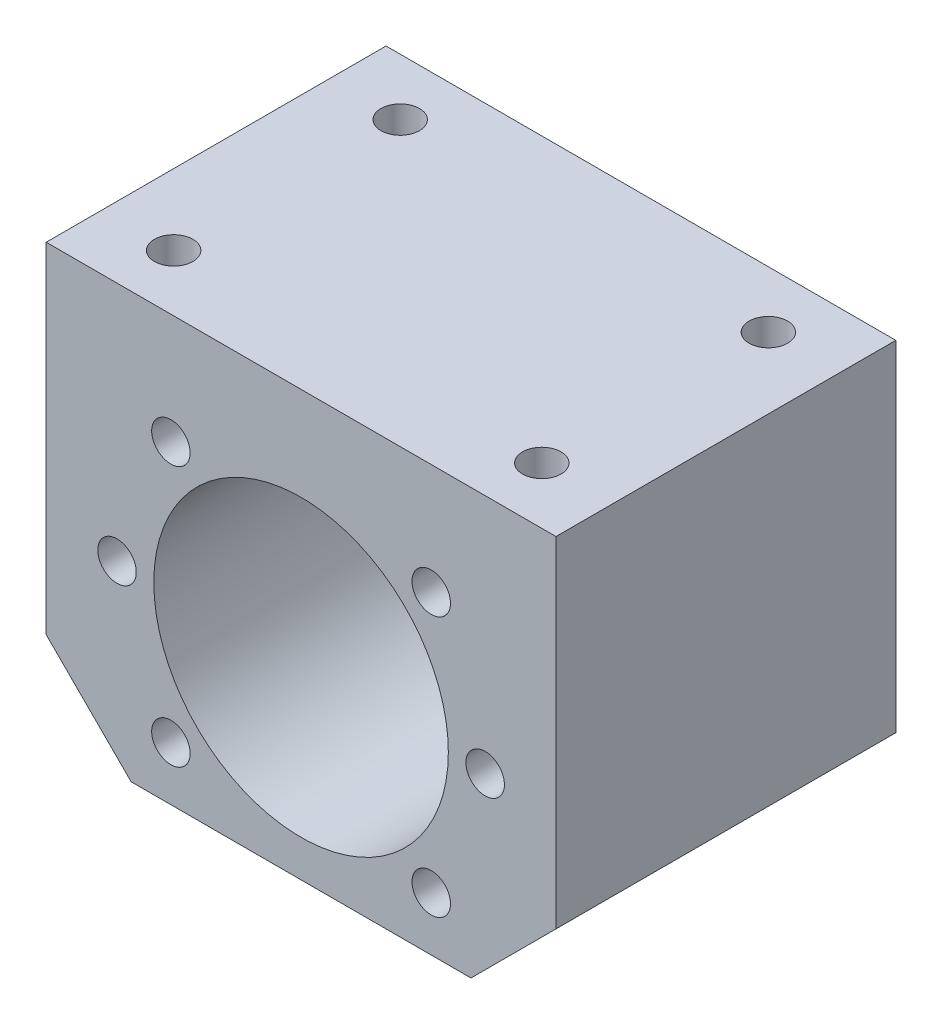
SolidWorks part; units mm, degrees
material "6061 合金"
ref_plane "前视基准面" through (0, 0, 0) normal (0, 0, 1) x (1, 0, 0)
ref_plane "上视基准面" through (0, 0, 0) normal (0, 1, 0) x (1, 0, 0)
ref_plane "右视基准面" through (0, 0, 0) normal (1, 0, 0) x (0, 0, -1)
sketch "草图1" plane through (0, 0, 0) normal (0, 0, 1) x (1, 0, 0)
  line L1 (45, -32.5) -> (-45, -32.5)
  line L2 (45, -32.5) -> (45, 42.5)
  line L3 (45, 42.5) -> (-45, 42.5)
  line L4 (-45, -32.5) -> (-45, 42.5)
  line L5 (45, -32.5) -> (-45, 42.5) construction
  line L6 (45, 42.5) -> (-45, -32.5) construction
  circle A1 centre (0, 0) radius 26
  point P1 (0, 5)
  dimension "D1" = 52
  dimension "D2" = 90
  dimension "D3" = 5
  dimension "D4" = 75
extrude "凸台-拉伸1" add sketch "草图1" along normal mid plane 60
sketch "草图2" plane through (0, 0, 30) normal (0, 0, 1) x (1, 0, 0)
  circle A0 centre (0, 0) radius 32.5
  point P3 (-32.5, 0)
  point P7 (-22.981, 22.981)
  point P8 (0, 32.5)
  point P9 (22.981, 22.981)
  point P10 (32.5, 0)
  point P11 (22.981, -22.981)
  point P12 (0, -32.5)
  point P13 (-22.981, -22.981)
  point P14 (0, 0)
  dimension "D1" = 65
  dimension "D2" = 8
hole_wizard "M8 螺纹孔1" positions "3D草图1" profile "草图3" tap size "M8" standard "GB"
sketch3d "3D草图1"
  point P0 (-32.5, 0, 30)
  point P3 (-22.981, 22.981, 30)
  point P6 (-22.981, -22.981, 30)
  point P9 (22.981, -22.981, 30)
  point P12 (32.5, 0, 30)
  point P15 (22.981, 22.981, 30)
sketch "草图3" plane through (-32.5, 0, 30) normal (1, 0, 0) x (0, -1, 0)
  line L0 (0, 0) -> (0, 21.7929)
  line L1 (0, 21.7929) -> (3.4, 19.75)
  line L2 (3.4, 19.75) -> (3.4, 0)
  line L5 (3.4, 0) -> (0, 0)
  line L10 (0, 21.7929) -> (-3.4, 19.75) construction
  line L11 (0, -6.35) -> (0, 107.95) construction
  dimension "螺纹孔钻头直径" = 6.8
  dimension "螺纹孔钻头深度" = 19.75
  dimension "导头角度" = 118
cosmetic thread "孔螺蚊线1" parameters "D1"=16, "D2"=8
cosmetic thread "孔螺蚊线2" parameters "D1"=16, "D2"=8
cosmetic thread "孔螺蚊线3" parameters "D1"=16, "D2"=8
cosmetic thread "孔螺蚊线4" parameters "D1"=16, "D2"=8
cosmetic thread "孔螺蚊线5" parameters "D1"=16, "D2"=8
cosmetic thread "孔螺蚊线6" parameters "D1"=16, "D2"=8
chamfer "倒角1" distance 15 angle 45 2 edges at (45, -32.5, 0) (-45, -32.5, 0)
sketch "草图4" plane through (0, 42.5, 0) normal (0, 1, 0) x (1, 0, 0)
  line L1 (32.5, -20) -> (-32.5, -20)
  line L2 (32.5, -20) -> (32.5, 20)
  line L3 (32.5, 20) -> (-32.5, 20)
  line L4 (-32.5, -20) -> (-32.5, 20)
  line L5 (32.5, -20) -> (-32.5, 20) construction
  line L6 (32.5, 20) -> (-32.5, -20) construction
  point P0 (0, 0)
  dimension "D1" = 65
  dimension "D2" = 40
hole_wizard "M8 螺纹孔2" positions "3D草图2" profile "草图5" tap size "M8" standard "GB"
sketch3d "3D草图2"
  point P2 (32.5, 42.5, -20)
  point P5 (32.5, 42.5, 20)
  point P8 (-32.5, 42.5, 20)
  point P11 (-32.5, 42.5, -20)
sketch "草图5" plane through (32.5, 42.5, -20) normal (1, 0, 0) x (0, 0, 1)
  line L0 (0, 0) -> (0, 21.7929)
  line L1 (0, 21.7929) -> (3.4, 19.75)
  line L2 (3.4, 19.75) -> (3.4, 0)
  line L5 (3.4, 0) -> (0, 0)
  line L10 (0, 21.7929) -> (-3.4, 19.75) construction
  line L11 (0, -6.35) -> (0, 107.95) construction
  dimension "螺纹孔钻头直径" = 6.8
  dimension "螺纹孔钻头深度" = 19.75
  dimension "导头角度" = 118
cosmetic thread "孔螺蚊线7" parameters "D1"=16, "D2"=8
cosmetic thread "孔螺蚊线8" parameters "D1"=16, "D2"=8
cosmetic thread "孔螺蚊线9" parameters "D1"=16, "D2"=8
cosmetic thread "孔螺蚊线10" parameters "D1"=16, "D2"=8
